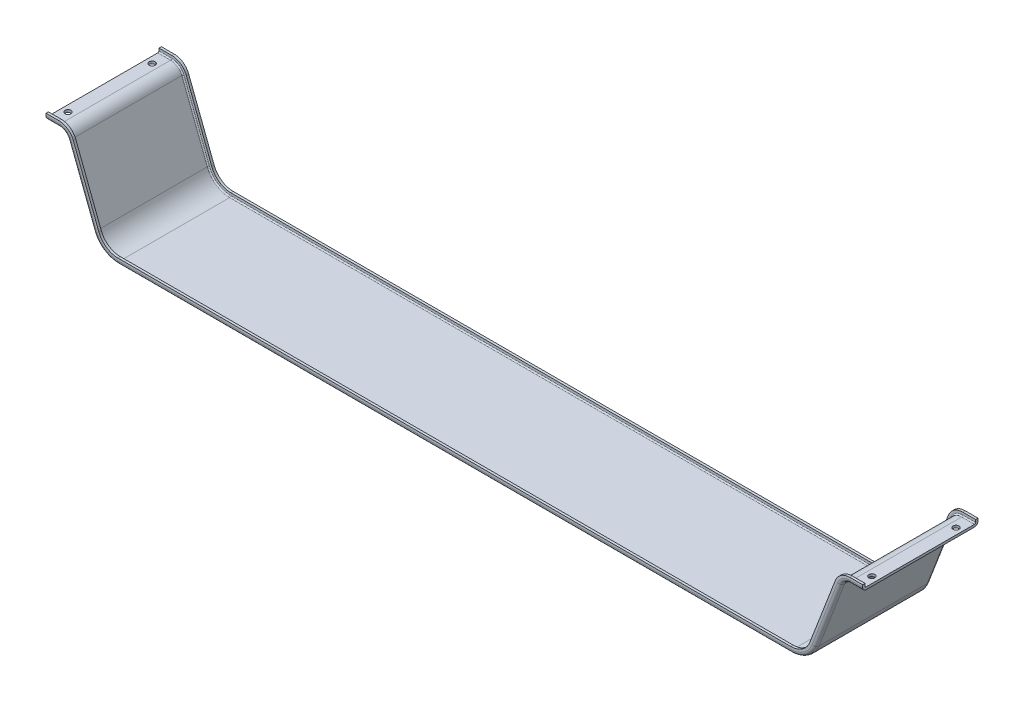
from build123d import *

# Parameters (mm, degrees)
SKETCH1_W                      = 1359.347595865
SKETCH1_H                      = 192
BOSS_EXTRUDE1_DEPTH            = 152.841538075
CUT_EXTRUDE1_DEPTH             = 184
SKETCH3_W                      = 1359.347595865
SKETCH3_H                      = 4
BOSS_EXTRUDE2_DEPTH            = 6
SKETCH4_W                      = 1359.347595865
SKETCH4_H                      = 4
BOSS_EXTRUDE3_DEPTH            = 6
CUT_EXTRUDE2_DEPTH             = 1510.687853091
CUT_EXTRUDE3_REACH             = 1511.688
CUT_EXTRUDE4_DEPTH             = 1510.687853091
CUT_EXTRUDE5_DEPTH             = 1510.184353805
F_10_0_10_DIAMETER_HOLE1_D     = 10
F_10_0_10_DIAMETER_HOLE1_DEPTH = 152.841538075
FILLET1_R                      = 34.000000002
FILLET2_R                      = 16
FILLET3_R                      = 20
FILLET4_R                      = 40.000000002
FILLET5_R                      = 44.000000002
FILLET6_R                      = 2
FILLET7_R                      = 6
FILLET8_R                      = 26


with BuildPart() as part:
    # Sketch1 → Boss-Extrude1 (new body)
    with BuildSketch(Plane(origin=(0, 107.054087174, 0), x_dir=(1, 0, 0), z_dir=(0, 1, 0))):
        with Locations((-813.481313616, 0)):
            Rectangle(SKETCH1_W, SKETCH1_H)
    extrude(amount=-BOSS_EXTRUDE1_DEPTH)

    # Sketch2 → Cut-Extrude1 (cut)
    with BuildSketch(Plane(origin=(0, 0, -92), x_dir=(-1, 0, 0), z_dir=(0, 0, -1))):
        Polygon((168.807515683, 107.054087174), (226, -41.787450901), (1400.962627231, -41.787450901), (1458.155111548, 107.054087174), align=None)
    extrude(amount=-CUT_EXTRUDE1_DEPTH, mode=Mode.SUBTRACT)

    # Sketch3 → Boss-Extrude2 (add)
    with BuildSketch(Plane(origin=(0, 107.054087174, 0), x_dir=(-1, 0, 0), z_dir=(0, 1, 0))):
        with Locations((813.481313616, -94)):
            Rectangle(SKETCH3_W, SKETCH3_H)
    extrude(amount=BOSS_EXTRUDE2_DEPTH)

    # Sketch4 → Boss-Extrude3 (add)
    with BuildSketch(Plane(origin=(0, 107.054087174, 0), x_dir=(-1, 0, 0), z_dir=(0, 1, 0))):
        with Locations((813.481313616, 94)):
            Rectangle(SKETCH4_W, SKETCH4_H)
    extrude(amount=BOSS_EXTRUDE3_DEPTH)

    # Sketch5 → Cut-Extrude2 (cut, through all)
    with BuildSketch(Plane(origin=(0, 0, -96), x_dir=(-1, 0, 0), z_dir=(0, 0, -1))):
        Polygon((166.059384321, 103.054087174), (133.807515683, 103.054087174), (133.807515683, -45.787450901), (223.251868638, -45.787450901), align=None)
    extrude(amount=-CUT_EXTRUDE2_DEPTH, mode=Mode.SUBTRACT)

    # Sketch6 → Cut-Extrude3 (cut, up to next)
    with BuildSketch(Plane(origin=(0, 0, -96), x_dir=(-1, 0, 0), z_dir=(0, 0, -1)), mode=Mode.PRIVATE) as cut_extrude3_sk1:
        Polygon((1454.032914506, 113.054087174), (172.929712725, 113.054087174), (230.122197042, -35.787450901), (1396.840430189, -35.787450901), align=None)
    cut_extrude3_tool1 = extrude(cut_extrude3_sk1.sketch, amount=-CUT_EXTRUDE3_REACH, mode=Mode.PRIVATE) & part.part
    add(cut_extrude3_tool1.solids().sort_by_distance((-813.481314, 39.792528, -96))[0], mode=Mode.SUBTRACT)

    # Sketch7 → Cut-Extrude4 (cut, through all)
    with BuildSketch(Plane.XY.offset(96)):
        Polygon((-1460.90324291, 103.054087174), (-1493.155111548, 103.054087174), (-1493.155111548, -45.787450901), (-1403.710758593, -45.787450901), align=None)
    extrude(amount=-CUT_EXTRUDE4_DEPTH, mode=Mode.SUBTRACT)

    # Sketch8 → Cut-Extrude5 (cut, through all)
    with BuildSketch(Plane(origin=(0, 0, 92), x_dir=(-1, 0, 0), z_dir=(0, 0, -1))):
        Polygon((1454.032914506, 113.054087174), (172.929712725, 113.054087174), (230.122197042, -35.787450901), (1396.840430189, -35.787450901), align=None)
    extrude(amount=-CUT_EXTRUDE5_DEPTH, mode=Mode.SUBTRACT)

    # Ø10.0 (10) Diameter Hole1
    with Locations(Plane(origin=(0, 107.054087174, 0), x_dir=(1, 0, 0), z_dir=(0, 1, 0))):
        with Locations((-144.437187279, 70), (-144.437187279, -70), (-1482.525439952, 70), (-1482.525439952, -70)):
            Hole(F_10_0_10_DIAMETER_HOLE1_D / 2, depth=F_10_0_10_DIAMETER_HOLE1_DEPTH)

    # Fillet1
    fillet1_edges = [part.edges().sort_by_distance(p)[0] for p in [
        (-1396.840430189, -35.787450901, 94),
        (-230.122197042, -35.787450901, 94),
        (-230.122197042, -35.787450901, -94),
        (-1396.840430189, -35.787450901, -94),
    ]]
    fillet(fillet1_edges, radius=FILLET1_R)

    # Fillet2
    fillet2_edges = [part.edges().sort_by_distance(p)[0] for p in [
        (-166.059384321, 103.054087174, 0),
        (-1460.90324291, 103.054087174, 0),
    ]]
    fillet(fillet2_edges, radius=FILLET2_R)

    # Fillet3
    fillet3_edges = [part.edges().sort_by_distance(p)[0] for p in [
        (-168.807515683, 107.054087174, 0),
        (-1458.155111548, 107.054087174, 0),
    ]]
    fillet(fillet3_edges, radius=FILLET3_R)

    # Fillet4
    fillet4_edges = [part.edges().sort_by_distance(p)[0] for p in [
        (-1400.962627231, -41.787450901, 0),
        (-226, -41.787450901, 0),
    ]]
    fillet(fillet4_edges, radius=FILLET4_R)

    # Fillet5
    fillet5_edges = [part.edges().sort_by_distance(p)[0] for p in [
        (-223.251868638, -45.787450901, 0),
        (-1403.710758593, -45.787450901, 0),
    ]]
    fillet(fillet5_edges, radius=FILLET5_R)

    # Fillet6
    fillet6_edges = [part.edges().sort_by_distance(p)[0] for p in [
        (-194.939490479, 39.04649198, -92),
        (-194.939490479, 39.04649198, 92),
        (-144.437187279, 107.054087174, -92),
        (-1482.525439952, 107.054087174, 92),
        (-166.39220553, 103.538519925, -92),
        (-166.39220553, 103.538519925, 92),
        (-1460.570421701, 103.538519925, -92),
        (-1460.570421701, 103.538519925, 92),
        (-1432.023136753, 39.04649198, -92),
        (-1432.023136753, 39.04649198, 92),
        (-813.481313616, -41.787450901, -92),
        (-230.830620305, -34.756316403, -92),
        (-1396.132006926, -34.756316403, -92),
        (-813.481313616, -41.787450901, 92),
        (-230.830620305, -34.756316403, 92),
        (-1396.132006926, -34.756316403, 92),
        (-1482.525439952, 107.054087174, -92),
        (-144.437187279, 107.054087174, 92),
    ]]
    fillet(fillet6_edges, radius=FILLET6_R)

    # Fillet7
    fillet7_edges = [part.edges().sort_by_distance(p)[0] for p in [
        (-144.437187279, 103.054087174, -96),
        (-144.437187279, 103.054087174, 96),
        (-1482.525439952, 103.054087174, 96),
        (-1482.525439952, 103.054087174, -96),
        (-164.127136199, 100.241633375, -96),
        (-164.127136199, 100.241633375, 96),
        (-1462.835491032, 100.241633375, 96),
        (-1462.835491032, 100.241633375, -96),
        (-1435.756975059, 37.611761518, 96),
        (-1435.756975059, 37.611761518, -96),
        (-813.481313616, -45.787450901, 96),
        (-191.205652172, 37.611761518, 96),
        (-228.565550974, -38.053202954, 96),
        (-1398.397076257, -38.053202954, 96),
        (-813.481313616, -45.787450901, -96),
        (-191.205652172, 37.611761518, -96),
        (-228.565550974, -38.053202954, -96),
        (-1398.397076257, -38.053202954, -96),
    ]]
    fillet(fillet7_edges, radius=FILLET7_R)

    # Fillet8
    fillet8_edges = [part.edges().sort_by_distance(p)[0] for p in [
        (-1454.032914506, 113.054087174, 94),
        (-172.929712725, 113.054087174, 94),
        (-172.929712725, 113.054087174, -94),
        (-1454.032914506, 113.054087174, -94),
    ]]
    fillet(fillet8_edges, radius=FILLET8_R)


solid = part.part
